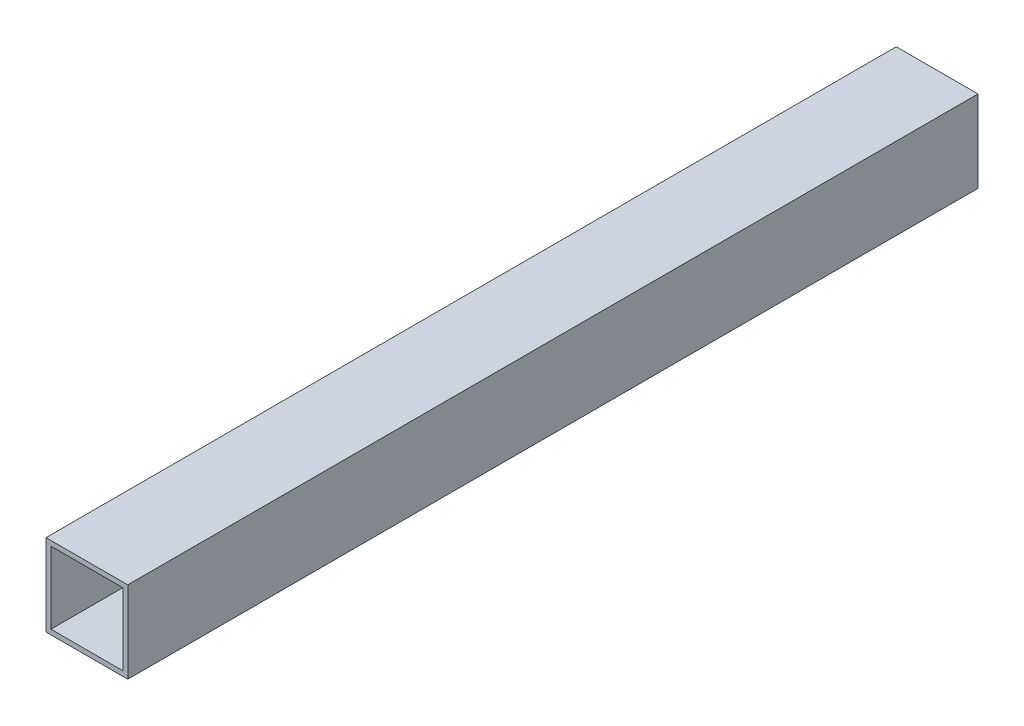
SolidWorks part; units mm, degrees
ref_plane "前视基准面" through (0, 0, 0) normal (0, 0, 1) x (1, 0, 0)
ref_plane "上视基准面" through (0, 0, 0) normal (0, 1, 0) x (1, 0, 0)
ref_plane "右视基准面" through (0, 0, 0) normal (1, 0, 0) x (0, 0, -1)
sketch "草图1" plane through (0, 0, 0) normal (0, 0, 1) x (1, 0, 0)
  line L0 (0, 0) -> (0, 50)
  line L1 (0, 50) -> (50, 50)
  line L2 (50, 50) -> (50, 0)
  line L3 (50, 0) -> (0, 0)
  line L4 (3, 3) -> (3, 47)
  line L5 (3, 47) -> (47, 47)
  line L6 (47, 47) -> (47, 3)
  line L7 (47, 3) -> (3, 3)
  dimension "D1" = 3
extrude "凸台-拉伸1" add sketch "草图1" along normal blind 520
